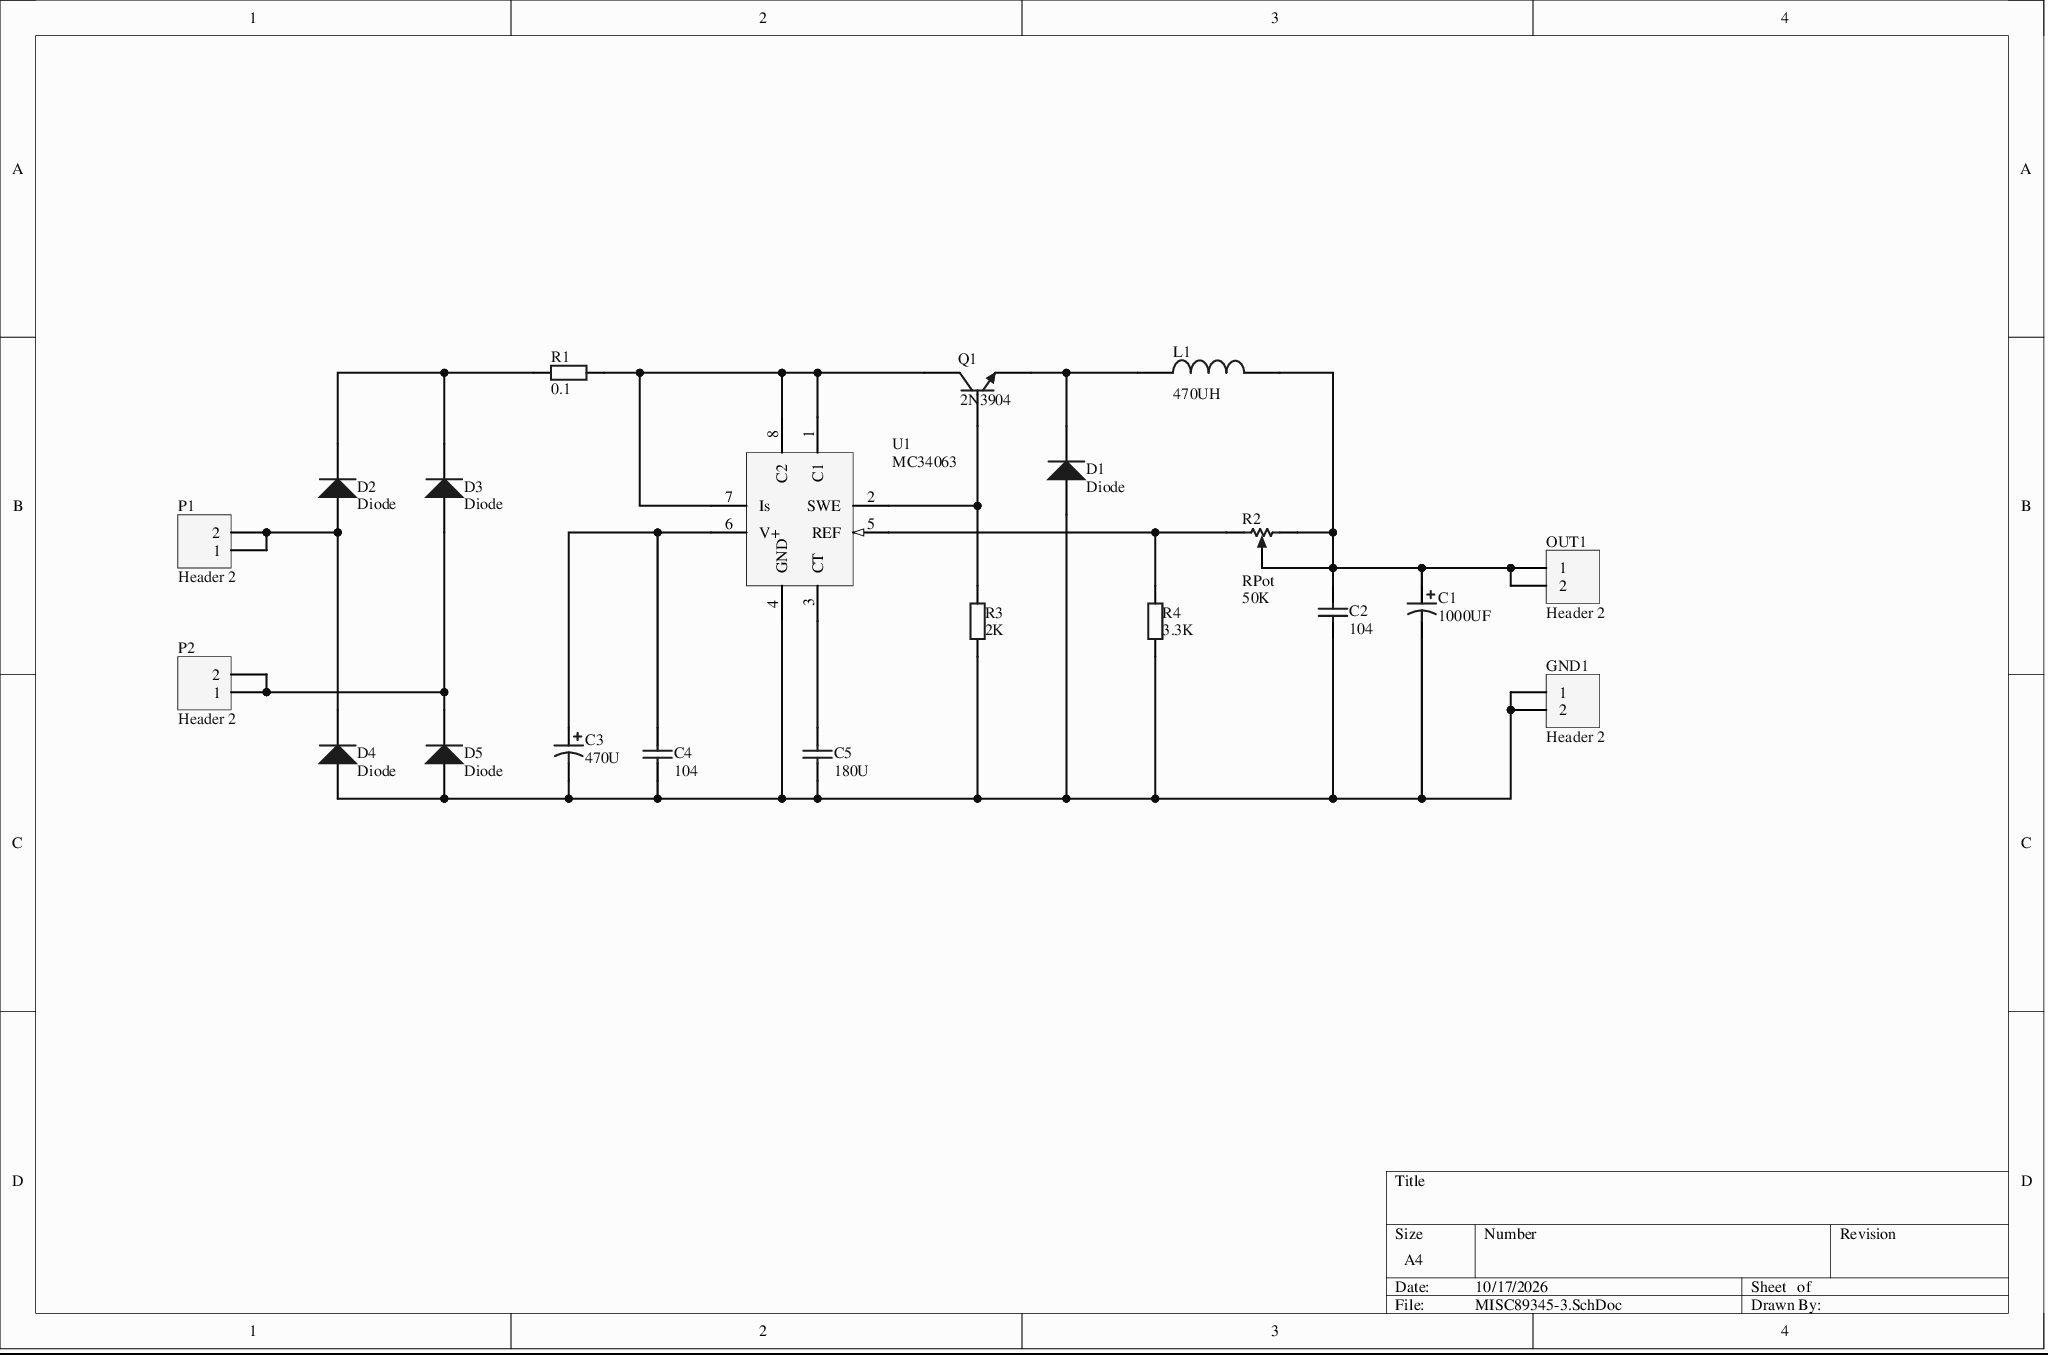
[diagram p0: MISC89345-3.SchDoc]
# Altium project MISC89345-6.PrjPcb
1 sheet, 21 parts. Net scope: global (net labels, ports and power ports of the same name join across sheets).
Board file: MISC89345.PcbDoc

## Sheet MISC89345-3.SchDoc
size A4

### Parts
C1  1000UF  [C0805]
C2  104  [C1206]
C3  470U  [C0805]
C4  104  [C1206]
C5  180U  [C1206]
D1  Diode  [SMC]
D2  Diode  [SMC]
D3  Diode  [SMC]
D4  Diode  [SMC]
D5  Diode  [SMC]
GND1  Header 2  [HDR1X2]
L1  470UH  [AL0204]
OUT1  Header 2  [HDR1X2]
P1  Header 2  [HDR1X2]
P2  Header 2  [HDR1X2]
Q1  2N3904  [TO-92A]
R1  0.1  [J1-0603]
R2  RPot  value 50K  [VR5]
R3  2K  [J1-0603]
R4  3.3K  [J1-0603]
U1  MC34063  [693-02]

### Nets
NetC1_1: C1.1 C2.2 L1.2 OUT1.1 OUT1.2 R2.2(BOT) R2.3(TAP)
NetC1_2: C1.2 C2.1 C3.2 C4.1 C5.1 D1.1(A) D4.1(A) D5.1(A) GND1.1 GND1.2 R3.1 R4.2 U1.4(GND)
NetC3_1: C3.1 C4.2 U1.6(V+)
NetC5_2: C5.2 U1.3(CT)
NetD1_2: D1.2(K) L1.1 Q1.1(E)
NetD2_1: D2.1(A) D4.2(K) P1.1 P1.2
NetD2_2: D2.2(K) D3.2(K) R1.2
NetD3_1: D3.1(A) D5.2(K) P2.1 P2.2
NetQ1_2: Q1.2(B) R3.2 U1.2(SWE)
NetQ1_3: Q1.3(C) R1.1 U1.1(C1) U1.7(Is) U1.8(C2)
NetR2_1: R2.1(TOP) R4.1 U1.5(REF)

### Library data of the parts
C1 C3 = Cap Pol3: Polarized Capacitor (Surface Mount); Value: 100pF; Published: 8-Jun-2000; LatestRevisionDate: 29-May-2009; LatestRevisionNote: IPC-7351 Footprint Added.; PackageReference: C0805; PackageDescription: Chip Capacitor; Publisher: Altium Limited
C2 C4 C5 = Cap Semi: Capacitor (Semiconductor SIM Model); Value: 100pF; Published: 8-Jun-2000; LatestRevisionDate: 29-May-2009; LatestRevisionNote: IPC-7351 Footprint Added.; PackageReference: C1206; PackageDescription: Chip Capacitor; Publisher: Altium Limited
D1-D5 = Diode: Default Diode; Published: 8-Jun-2000; LatestRevisionDate: 17-Jul-2002; LatestRevisionNote: Re-released for DXP Platform.; PackageVersion: Sep-1996; PackageReference: SMC; PackageDescription: DO-214-AB/SMC; 2 C-Bend Leads; Body 7.9 x 5.9 mm, inc. leads (LxW); Code_JEDEC: DO-214-AB; Publisher: Altium Limited
GND1 OUT1 P1 P2 = Header 2: Header, 2-Pin; LatestRevisionDate: 17-Jul-2002; LatestRevisionNote: Re-released for DXP Platform.; Publisher: Altium Limited
L1 = INDUCTOR
Q1 = 2N3904: NPN General Purpose Amplifier; Published: 8-Jun-2000; LatestRevisionDate: 15-Jan-2003; LatestRevisionNote: PCB Footprint 'BCY-W3/D4.7' replaced; DatasheetVersion: 1997; PackageVersion: Sep-1998; PackageReference: TO-92A; PackageDescription: TO, Flat Index; 3 In-Line, Axial Leads; Body Dia. 4.5mm; Leads 0.51 x 0.48 mm (max); ComponentLink1Description: Manufacturer Link; ComponentLink2Description: Datasheet; ComponentLink2URL: http://example.com/ds/2N%2F2N3904.pdf; Publisher: Altium Limited
R1 R3 R4 = Res2: Resistor; Value: 1K; Published: 8-Jun-2000; LatestRevisionDate: 17-Jul-2002; LatestRevisionNote: Re-released for DXP Platform.; PackageReference: AXIAL-0.4; PackageDescription: Axial Device, Thru-Hole; 2 Leads; 0.4 in Pin Spacing; Publisher: Altium Limited
R2 = RPot: Potentiometer; Sim Note: Enter the Resistance value and the set point into parameter fields.; Set Position: 0.5; Published: 8-Jun-2000; LatestRevisionDate: 17-Jul-2002; LatestRevisionNote: Re-released for DXP Platform.; PackageReference: VR5; PackageDescription: Variable Resistor, Thru-Hole; 3 Leads; Publisher: Altium Limited
U1 = MC34063U: DC-to-DC Converter Control Circuit; Code - JEDEC: MO-001-AN; Published: 17-Jul-2002; Datasheet: Linear and Interface Integrated Circuits, DL128 Rev2 (1988); Package Reference: 693-02; Publisher: Altium Limited